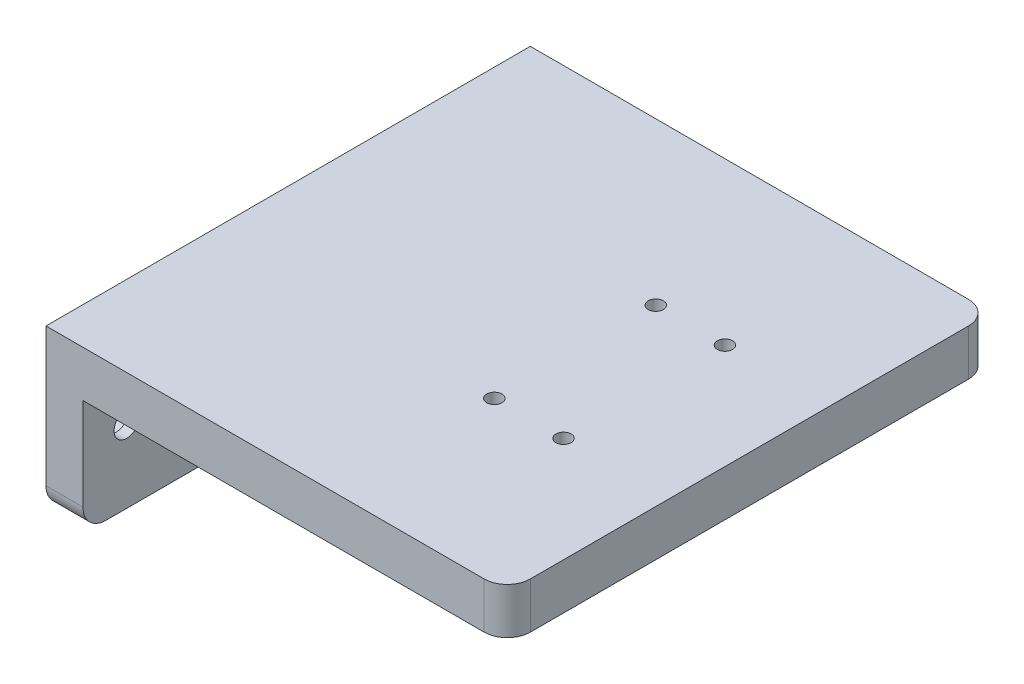
SolidWorks part; units mm, degrees
material "6061 合金"
ref_plane "前视" through (0, 0, 0) normal (0, 0, 1) x (1, 0, 0)
ref_plane "上视" through (0, 0, 0) normal (0, 1, 0) x (1, 0, 0)
ref_plane "右视" through (0, 0, 0) normal (1, 0, 0) x (0, 0, -1)
sketch "草图1" plane through (0, 0, 0) normal (0, 0, 1) x (1, 0, 0)
  line L0 (0, 0) -> (0, 50)
  line L1 (0, 0) -> (90, 0)
  dimension "D1" = 50
  dimension "D2" = 90
extrude "拉伸-薄壁1" add sketch "草图1" along normal mid plane 54 thin thin type one direction wall 10
sketch "草图2" plane through (0, 0, 0) normal (1, 0, 0) x (0, 0, -1)
  line L0 (0, 0) -> (0, 30) construction
  line L1 (-27, -10) -> (27, -10) construction
  circle A0 centre (0, 30) radius 16
  dimension "D1" = 32
  dimension "D2" = 40
extrude "切除-拉伸1" cut sketch "草图2" against normal through all
sketch "草图3" plane through (-10, 0, 0) normal (-1, 0, 0) x (0, 0, 1)
  circle A0 centre (0, 30) radius 15
  circle A1 centre (0, 30) radius 16 construction
  circle A2 centre (0, 30) radius 16
  dimension "D1" = 30
extrude "凸台-拉伸1" add sketch "草图3" against normal blind 1.2
sketch "草图5" plane through (0, 0, 0) normal (0, 1, 0) x (1, 0, 0)
  line L0 (90, -27) -> (90, 27) construction
  line L1 (-10, -52.5) -> (90, -52.5)
  line L2 (-10, -52.5) -> (-10, 52.5)
  line L3 (-10, 52.5) -> (90, 52.5)
  line L4 (90, -52.5) -> (90, 52.5)
  line L5 (-10, -52.5) -> (90, 52.5) construction
  line L6 (-10, 52.5) -> (90, -52.5) construction
  line L7 (0, 0) -> (70.3449, 0) construction
  line L8 (0, -27) -> (0, 27) construction
  line L9 (-10, -27) -> (-10, 27) construction
  point P0 (40, 0)
  dimension "D2" = 105
extrude "凸台-拉伸2" add sketch "草图5" against normal up to surface (10 mm away) up to face at (40, -10, 0)
fillet "圆角1" radius 5 4 edges at (90, -5, -52.5) (90, -5, 52.5) (-5, 50, -27) (-5, 50, 27)
sketch "草图6" plane through (0, 0, 0) normal (0, 1, 0) x (1, 0, 0)
  line L0 (0, 0) -> (90, 0) construction
  line L1 (90, -47.5) -> (90, 47.5) construction
  line L3 (0, -43) -> (72, -43)
  line L4 (0, -43) -> (0, 43)
  line L5 (0, 43) -> (72, 43)
  line L6 (72, -43) -> (72, 43)
  line L7 (0, -43) -> (72, 43) construction
  line L8 (0, 43) -> (72, -43) construction
  dimension "D1" = 72
  dimension "D2" = 86
  dimension "D3" = 18
sketch "草图8" plane through (0, 0, 0) normal (0, 1, 0) x (1, 0, 0)
  point P0 (67.2, -17.5)
  point P1 (52.2, -17.5)
  point P3 (67.2, 17.5)
  point P5 (52.2, 17.5)
hole_wizard "M4 螺纹孔1" positions "3D草图2" profile "草图9" tap size "M4" standard "GB" end condition through all
sketch3d "3D草图2"
  point P0 (67.2, 0, 17.5)
  point P3 (52.2, 0, 17.5)
  point P6 (67.2, 0, -17.5)
  point P9 (52.2, 0, -17.5)
sketch "草图9" plane through (67.2, 0, 17.5) normal (1, 0, 0) x (0, 0, 1)
  line L0 (0, 0) -> (0, 10)
  line L1 (0, 10) -> (1.65, 10)
  line L2 (1.65, 10) -> (1.65, 0)
  line L5 (1.65, 0) -> (0, 0)
  line L11 (0, -6.35) -> (0, 107.95) construction
  dimension "通孔螺纹孔钻头直径" = 3.3
  dimension "通孔螺纹孔钻头深度" = 10
cosmetic thread "孔螺蚊线1" parameters "D2"=4
cosmetic thread "孔螺蚊线2" parameters "D2"=4
cosmetic thread "孔螺蚊线3" parameters "D2"=4
cosmetic thread "孔螺蚊线4" parameters "D2"=4
sketch "草图10" plane through (0, 50, 0) normal (0, 1, 0) x (1, 0, 0)
  line L1 (-16.2443, 28.7831) -> (5.6252, 28.7831)
  line L2 (-16.2443, 28.7831) -> (-16.2443, -29.7707)
  line L3 (-16.2443, -29.7707) -> (5.6252, -29.7707)
  line L4 (5.6252, 28.7831) -> (5.6252, -29.7707)
extrude "切除-拉伸2" cut sketch "草图10" against normal up to surface (50 mm away) up to face at (67.2, 0, 19.15)
sketch "草图11" plane through (-10, 0, 0) normal (-1, 0, 0) x (0, 0, 1)
  line L0 (-52.5, 0) -> (52.5, 0) construction
  line L1 (-52.5, 0) -> (52.5, 0)
  line L2 (-52.5, 0) -> (-52.5, -35)
  line L3 (-52.5, -35) -> (52.5, -35)
  line L4 (52.5, 0) -> (52.5, -35)
  line L5 (52.5, -10) -> (52.5, 0) construction
  dimension "D1" = 35
extrude "凸台-拉伸3" add sketch "草图11" against normal blind 8
sketch "草图12" plane through (-10, 0, 0) normal (-1, 0, 0) x (0, 0, 1)
  line L0 (0, 0) -> (0, -37.0158) construction
  line L1 (-43, -19.1) -> (-11, -19.1) construction
  line L2 (43, -19.1) -> (11, -19.1) construction
  line L3 (-52.5, -10) -> (52.5, -10) construction
  dimension "D1" = 22
  dimension "D2" = 86
  dimension "D3" = 9.1
hole_wizard "M5 六角圆柱头螺钉的柱形沉头孔1" positions "3D草图3" profile "草图13" counterbore size "M5" standard "GB"
sketch3d "3D草图3"
  point P0 (-10, -19.1, -43)
  point P3 (-10, -19.1, -11)
  point P6 (-10, -19.1, 11)
  point P9 (-10, -19.1, 43)
sketch "草图13" plane through (-10, -19.1, -43) normal (0, 1, 0) x (0, 0, 1)
  line L0 (0, 0) -> (0, 11.7524)
  line L1 (0, 11.7524) -> (2.75, 10.1)
  line L2 (2.75, 10.1) -> (2.75, 5.7)
  line L3 (2.75, 5.7) -> (5, 5.7)
  line L4 (5, 5.7) -> (5, 0)
  line L5 (5, 0) -> (0, 0)
  line L10 (0, 11.7524) -> (-2.75, 10.1) construction
  line L11 (0, -6.35) -> (0, 107.95) construction
  dimension "孔直径" = 5.5
  dimension "孔深度" = 10.1
  dimension "柱形沉头孔直径" = 10
  dimension "柱形沉头孔深度" = 5.7
  dimension "导头角度" = 118
fillet "圆角2" radius 5 2 edges at (-6, -35, -52.5) (-6, -35, 52.5)
